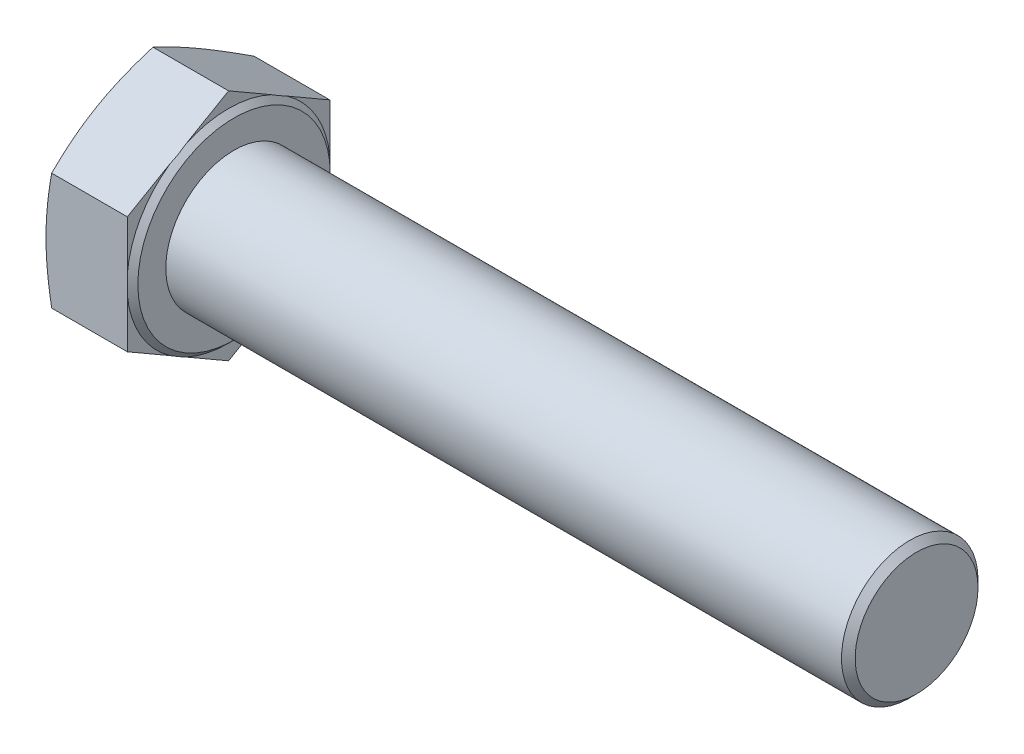
SolidWorks part; units mm, degrees
ref_plane "Front" through (0, 0, 0) normal (0, 0, 1) x (1, 0, 0)
ref_plane "Top" through (0, 0, 0) normal (0, 1, 0) x (1, 0, 0)
ref_plane "Right" through (0, 0, 0) normal (1, 0, 0) x (0, 0, -1)
other "Configuration Table"
sketch "Sketch2" plane through (0, 0, 0) normal (1, 0, 0) x (0, 0, -1)
  line L1 (14.835, -8.565) -> (14.835, 8.565)
  line L2 (14.835, 8.565) -> (0, 17.13)
  line L3 (0, 17.13) -> (-14.835, 8.565)
  line L4 (-14.835, 8.565) -> (-14.835, -8.565)
  line L5 (-14.835, -8.565) -> (0, -17.13)
  line L6 (0, -17.13) -> (14.835, -8.565)
  circle A0 centre (0, 0) radius 14.835 construction
extrude "BaseHead" add sketch "Sketch2" along normal blind 12.715
sketch "Sketch3" plane through (0, 0, 0) normal (0, 0, 1) x (1, 0, 0)
  line L0 (12.715, 17.13) -> (12.715, 14.095)
  line L2 (12.715, 14.095) -> (11.915, 14.895)
  line L3 (11.915, 14.895) -> (11.915, 17.13)
  line L5 (11.915, 17.13) -> (12.715, 17.13)
  line L6 (-0.9571, 0) -> (7.6478, 0) construction
  line L7 (12.715, 17.13) -> (0, 17.13) construction
  dimension "D1" = 45
  dimension "c" = 0.8
  dimension "Dw" = 28.19
revolve "BearingFace" cut sketch "Sketch3" angle 360 about L6
sketch "Sketch4" plane through (0, 0, 0) normal (0, 0, 1) x (1, 0, 0)
  line L0 (-0.4935, 0) -> (3.5626, 0) construction
  line L2 (0, 17.13) -> (0.8353, 17.13)
  line L4 (0.8353, 17.13) -> (0, 14.835)
  line L6 (0, 14.835) -> (0, 17.13)
  line L7 (11.915, 17.13) -> (0, 17.13) construction
revolve "HeadChamfer" cut sketch "Sketch4" angle 360 about L0
sketch "Sketch5" plane through (12.715, 0, 0) normal (1, 0, 0) x (0, 0, -1)
  circle A0 centre (0, 0) radius 10
extrude "BaseBody" add sketch "Sketch5" along normal blind 100
cosmetic thread "ThreadCosmetic1" [suppressed] parameters "D2"=17.294
chamfer "Chamfer1" distance 1 angle 45 1 edges at (112.715, 0, -10)
fillet "HeadFillet" [suppressed] radius 0.8
sketch "Sketch6" plane through (0, 0, 0) normal (0, 0, 1) x (1, 0, 0)
  line L0 (12.715, 11.353) -> (14.068, 11.353)
  line L1 (14.068, 11.353) -> (14.068, 10)
  line L2 (14.068, 10) -> (13.3915, 8.8283)
  line L3 (13.3915, 8.8283) -> (12.715, 10)
  line L4 (12.715, 10) -> (12.715, 11.353)
  line L5 (111.715, 10) -> (12.715, 10) construction
  line L6 (12.715, -14.095) -> (12.715, 14.095) construction
revolve "Cut-Revolve10" [suppressed] cut sketch "Sketch6" angle 360 about axis through (-0.9571, 0, 0) along (1, 0, 0)
pattern_linear "LPattern10" [suppressed] count 62
equation "\"D2@Sketch4\" = \"s@Sketch2\""
equation "\"D1@Chamfer1\" = 0.05 * \"d@Sketch5\""
equation "\"D1@Sketch6\" =  ( \"d@Sketch5\" - \"D2@ThreadCosmetic1\" )  / 2"
equation "\"pitch@LPattern10\" = \"D1@Sketch6\" * 1.2"
equation "\"D1@LPattern10\" = \"l@BaseBody\" / \"pitch@LPattern10\""
